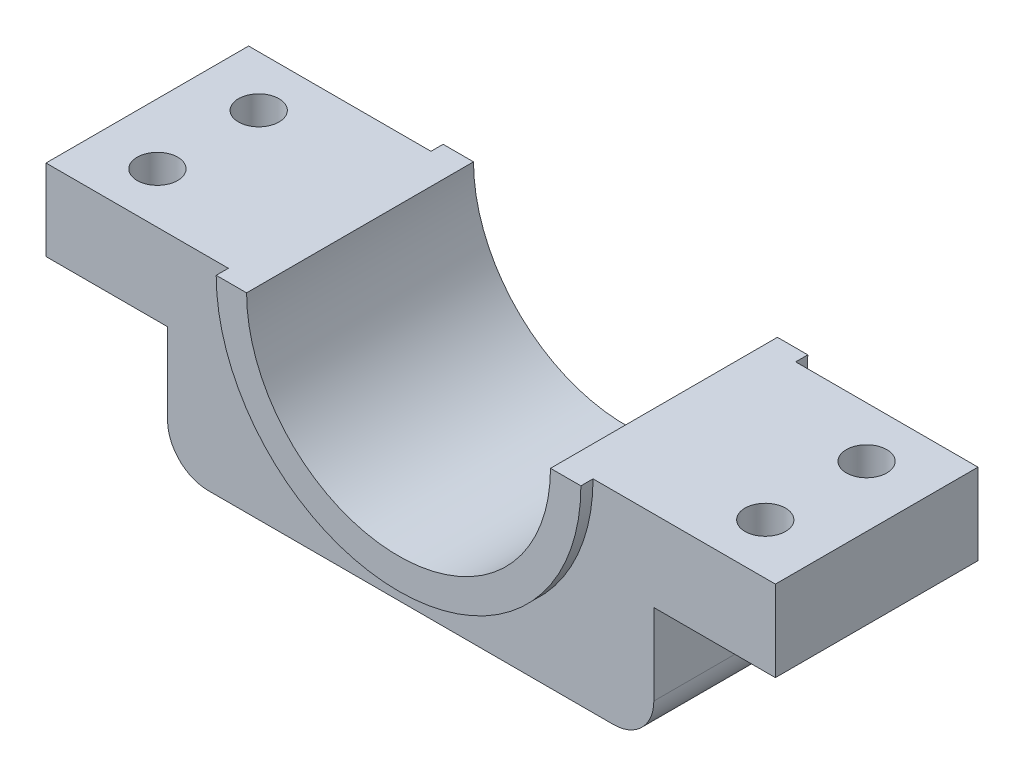
SolidWorks part; units mm, degrees
ref_plane "前视基准面" through (0, 0, 0) normal (0, 0, 1) x (1, 0, 0)
ref_plane "上视基准面" through (0, 0, 0) normal (0, 1, 0) x (1, 0, 0)
ref_plane "右视基准面" through (0, 0, 0) normal (1, 0, 0) x (0, 0, -1)
other "Configuration Table"
sketch "草图1" plane through (0, 0, 0) normal (0, 1, 0) x (1, 0, 0)
  line L1 (-60, -25) -> (60, -25)
  line L2 (-60, -25) -> (-60, 25)
  line L3 (-60, 25) -> (60, 25)
  line L4 (60, -25) -> (60, 25)
  line L5 (-60, -25) -> (60, 25) construction
  line L6 (-60, 25) -> (60, -25) construction
  point P0 (0, 0)
  dimension "D1" = 120
  dimension "D2" = 50
extrude "凸台-拉伸1" add sketch "草图1" against normal blind 50 contours L1 L4 L3 L2
sketch "草图2" plane through (0, 0, 25) normal (0, 0, 1) x (1, 0, 0)
  circle A0 centre (0, 0) radius 37.5
  dimension "D1" = 75
extrude "切除-拉伸1" cut sketch "草图2" against normal blind 50 contours A0
sketch "草图3" plane through (0, 0, 0) normal (0, -1, 0) x (1, 0, 0)
  line L0 (-60, 25) -> (60, 25) construction
  line L1 (-90, -25) -> (-60, -25)
  line L2 (-90, -25) -> (-90, 25)
  line L3 (-90, 25) -> (-60, 25)
  line L4 (90, -25) -> (90, 25)
  line L5 (-90, -25) -> (90, 25) construction
  line L6 (-90, 25) -> (90, -25) construction
  line L7 (-60, 25) -> (-60, -25) construction
  line L8 (60, 25) -> (60, -25) construction
  line L9 (-60, 25) -> (-60, -25)
  line L10 (60, 25) -> (60, -25)
  line L11 (60, 25) -> (90, 25)
  line L12 (60, -25) -> (90, -25)
  point P0 (0, 0)
  dimension "D1" = 180
extrude "凸台-拉伸3" add sketch "草图3" along normal blind 20
fillet "圆角1" radius 10 2 edges at (60, -50, 0) (-60, -50, 0)
sketch "草图5" plane through (0, 0, 0) normal (0, 1, 0) x (1, 0, 0)
  line L0 (-90, -25) -> (-37.5, -25) construction
  line L1 (-90, 25) -> (-37.5, 25) construction
  line L2 (0, 0) -> (0, 32.3741) construction
  circle A0 centre (-75, 12.5) radius 5
  circle A1 centre (-75, -12.5) radius 5
  circle A2 centre (75, -12.5) radius 5
  circle A3 centre (75, 12.5) radius 5
  dimension "D2" = 10
  dimension "D1" = 75
  dimension "D3" = 12.5
  dimension "D4" = 12.5
extrude "切除-拉伸2" cut sketch "草图5" against normal blind 20
sketch "草图6" plane through (0, 0, 25) normal (0, 0, 1) x (1, 0, 0)
  line L0 (-45, 0) -> (-37.5, 0)
  line L3 (37.5, 0) -> (45, 0)
  arc A0 (-37.5, 0) -> (37.5, 0) centre (0, 0) ccw construction
  arc A1 (-37.5, 0) -> (37.5, 0) centre (0, 0) ccw
  arc A2 (-45, 0) -> (45, 0) centre (0, 0) ccw
  dimension "D1" = 90
extrude "凸台-拉伸4" add sketch "草图6" along normal blind 3
mirror "镜向1" about plane through (0, 0, 0) normal (0, 0, 1) of "凸台-拉伸4"
